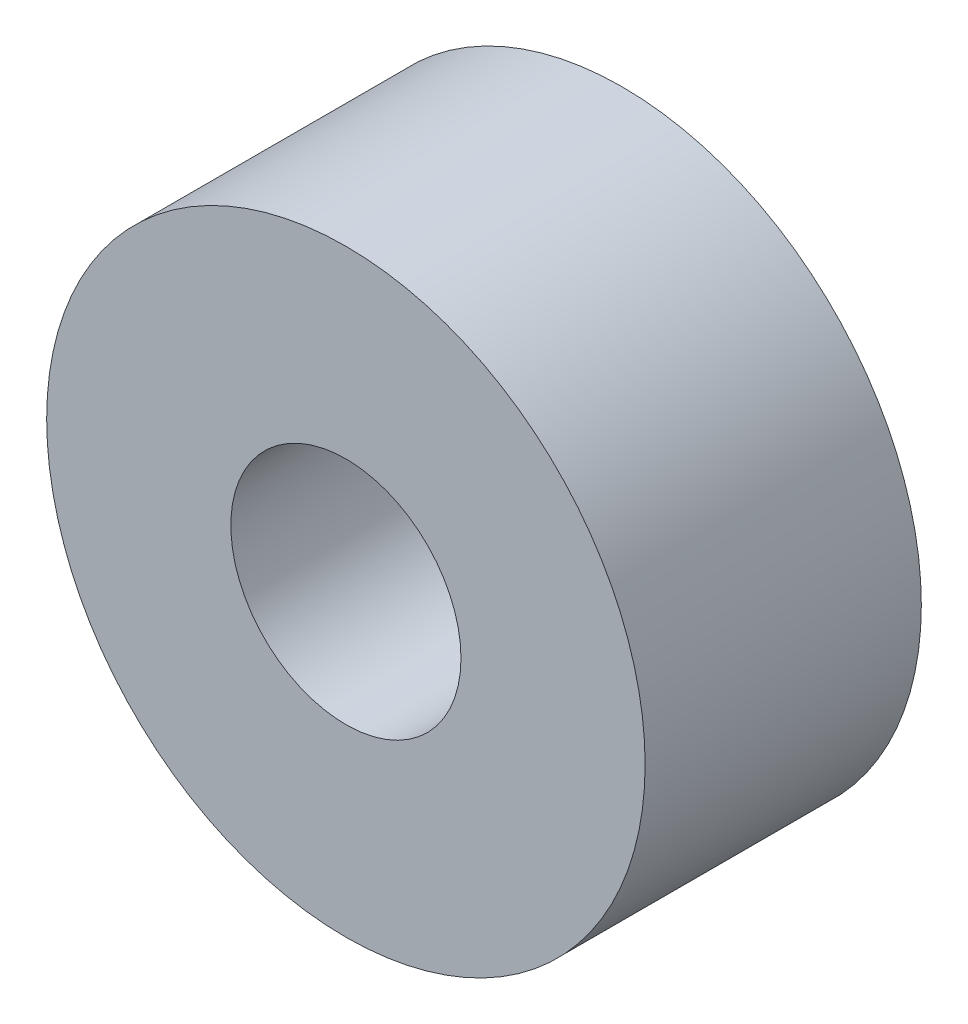
from build123d import *

# Parameters (mm, degrees)
SKETCH2_R           = 6.5
SKETCH2_R_2         = 2.5
BOSS_EXTRUDE1_DEPTH = 6


with BuildPart() as part:
    # Sketch2 → Boss-Extrude1 (new body)
    with BuildSketch(Plane.XY):
        Circle(SKETCH2_R)
        Circle(SKETCH2_R_2, mode=Mode.SUBTRACT)
    extrude(amount=BOSS_EXTRUDE1_DEPTH)


solid = part.part
